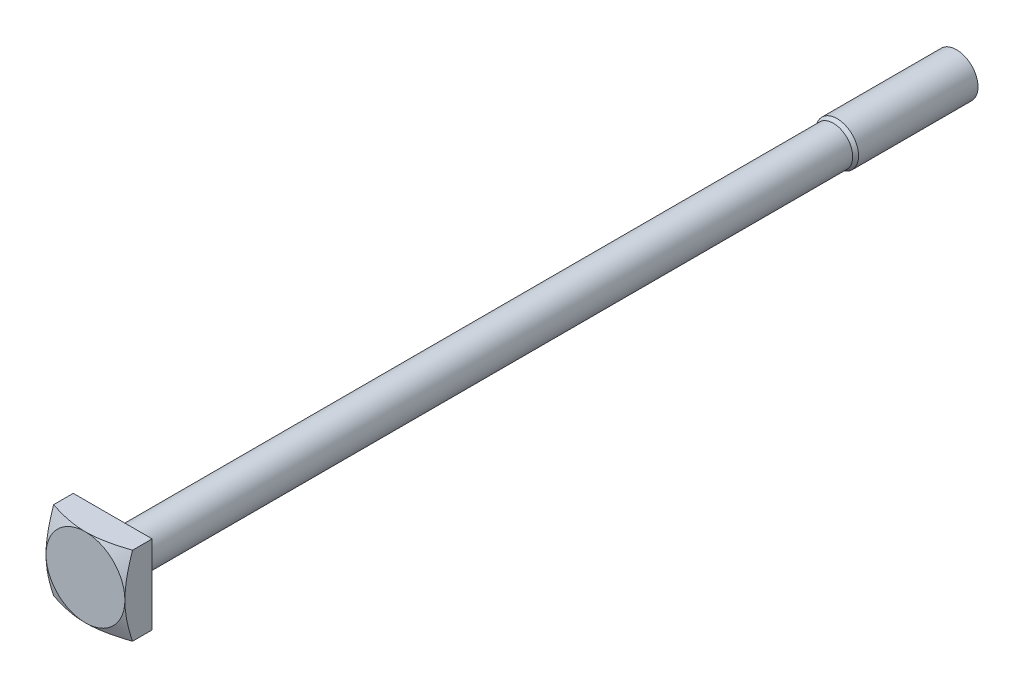
SolidWorks part; units mm, degrees
extrude "Base-Extrude" add sketch "Sketch1" along normal blind 19
sketch "Sketch1" plane through (0, 0, 0) normal (0, 0, 1) x (1, 0, 0)
  line L0 (-27.5, 27.5) -> (27.5, -27.5) construction
  line L1 (-27.5, 27.5) -> (27.5, 27.5)
  line L2 (-27.5, 27.5) -> (-27.5, -27.5)
  line L3 (-27.5, -27.5) -> (27.5, -27.5)
  line L4 (27.5, 27.5) -> (27.5, -27.5)
  dimension "D1" = 55
revolve "Boss-Revolve1" add sketch "Sketch2" angle 360 about L6
sketch "Sketch2" plane through (0, 0, 0) normal (0, 1, 0) x (1, 0, 0)
  line L0 (0, 0) -> (13.5, 0)
  line L1 (27.5, 0) -> (-27.5, 0) construction
  line L2 (13.5, 0) -> (13.5, 502.4019)
  line L3 (13.5, 502.4019) -> (15, 505)
  line L4 (15, 505) -> (15, 590)
  line L5 (15, 590) -> (0, 590)
  line L6 (0, 590) -> (0, 0) construction
  line L7 (0, 0) -> (0, 590)
cosmetic thread "Thread1" parameters "D1"=86.299, "D2"=26.969
ref_plane "front" through (0, 0, 0) normal (0, 0, 1) x (1, 0, 0)
ref_plane "top" through (0, 0, 0) normal (0, 1, 0) x (1, 0, 0)
ref_plane "right" through (0, 0, 0) normal (1, 0, 0) x (0, 0, -1)
sketch "dimension sketch" plane through (0, 0, 0) normal (0, 1, 0) x (1, 0, 0)
  line L0 (-29.25, 0) -> (29.25, 0)
  line L1 (29.25, 0) -> (29.25, 19)
  line L2 (29.25, 19) -> (14.1134, 19)
  line L3 (13.1134, 20) -> (13.1134, 515.2)
  line L4 (13.1134, 515.2) -> (15, 524)
  line L5 (15, 524) -> (15, 609)
  line L6 (15, 609) -> (-15, 609)
  line L7 (0, 0) -> (0, 609) construction
  line L8 (-29.25, 19) -> (-14.1134, 19)
  line L9 (-29.25, 0) -> (-29.25, 19)
  line L10 (-15, 524) -> (-15, 609)
  line L11 (-13.1134, 515.2) -> (-15, 524)
  line L12 (-13.1134, 20) -> (-13.1134, 515.2)
  arc A0 (14.1134, 19) -> (13.1134, 20) centre (14.1134, 20) cw
  arc A1 (-14.1134, 19) -> (-13.1134, 20) centre (-14.1134, 20) ccw
  point P9 (4.1274, 46)
  point P10 (15, 612.5)
sketch "Sketch4" plane through (0, 0, 19) normal (0, 0, 1) x (1, 0, 0)
  line L0 (27.5, 27.5) -> (-27.5, 27.5) construction
  circle A0 centre (0, 0) radius 27.5
extrude "Cut-Extrude1" cut sketch "Sketch4" against normal through all draft 65 flip side to cut
fillet "Fillet1" radius 1 1 edges at (13.5, 0, 0)
sketch "Sketch3" plane through (0, 0, 0) normal (0, 1, 0) x (1, 0, 0)
  line L0 (11.969, 590) -> (15, 591.7499)
  line L1 (15, 590) -> (-15, 590) construction
  line L2 (15, 591.7499) -> (15, 588.2501)
  line L3 (15, 588.2501) -> (11.969, 590)
  line L4 (0, 0) -> (0, 4.1158) construction
  line L5 (0, 590) -> (0, 0) construction
  line L6 (15, 505) -> (15, 590) construction
revolve "Cut-Revolve1" cut sketch "Sketch3" angle 360 about L4
pattern_linear "LPattern1" [suppressed] count 25 spacing 3.5
equation "\"D1@Base-Extrude\" = \"K@dimension sketch\""
equation "\"D1@Fillet1\" = \"r@dimension sketch\""
equation "\"D1@Sketch2\" = \"x@dimension sketch\""
equation "\"D2@Sketch2\"= \"L@dimension sketch\" "
equation "\"D4@Sketch2\"=\"B@dimension sketch\" "
equation "\"D3@Sketch2\" = \"D@dimension sketch\"/2"
equation "\"D3@LPattern1\" = \"P@dimension sketch\""
equation "\"D5@Sketch2\" = \"D3@Sketch2\" * 2 -3"
equation "\"D1@LPattern1\" = \"D4@Sketch2\" / \"D3@LPattern1\"+1"
equation "\"D3@Sketch3\" = \"D3@LPattern1\"*0.866"
equation "\"D1@Thread1\" = \"D4@Sketch2\" + \"D1@Sketch2\" / 2"
equation "\"D2@Thread1\" = \"D3@Sketch2\" * 2 - \"D3@Sketch3\""
